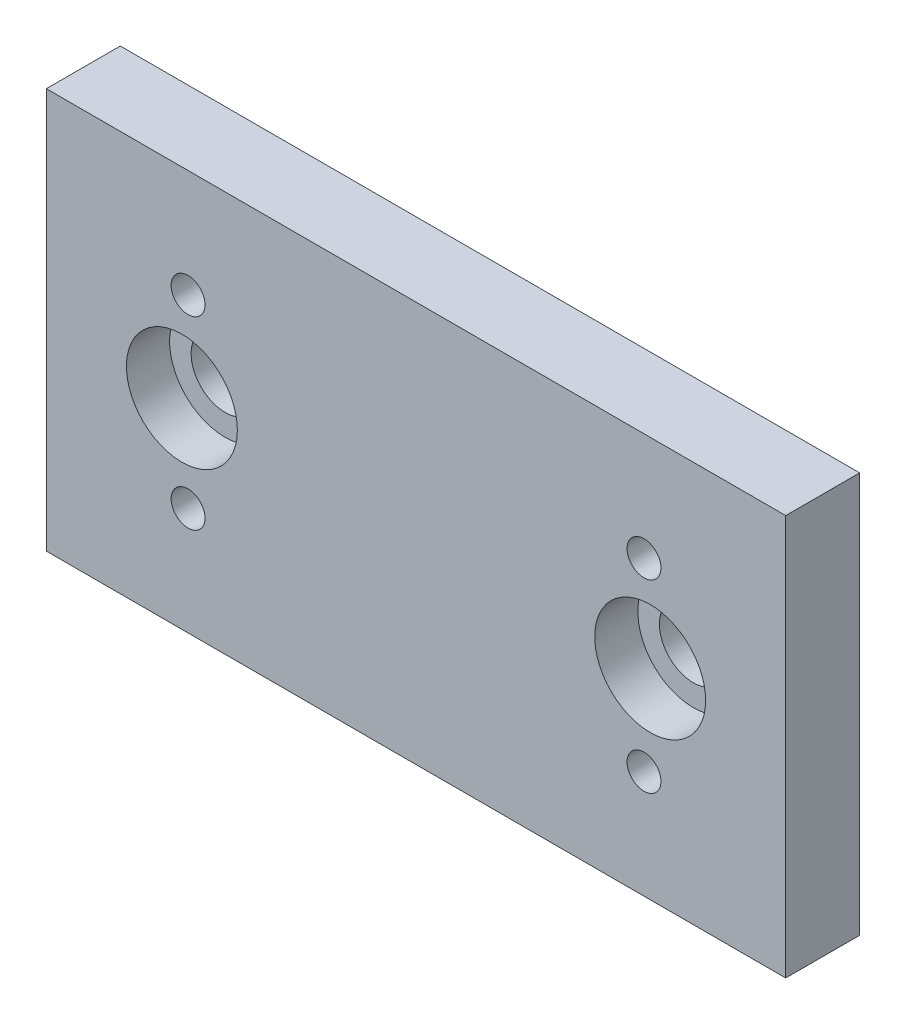
from build123d import *

# Parameters (mm, degrees)
SKETCH1_W                                        = 120
SKETCH1_H                                        = 65
BOSS_EXTRUDE1_DEPTH                              = 12
HOLE_FOR_TORX_SOCKET_CAP_SCREW1_D                = 11
HOLE_FOR_TORX_SOCKET_CAP_SCREW1_CBORE_D          = 18
HOLE_FOR_TORX_SOCKET_CAP_SCREW1_CBORE_DEPTH      = 7
HOLE_FOR_SOCKET_HEAD_CAP_SCREW_TYPE2_D           = 5.5
HOLE_FOR_SOCKET_HEAD_CAP_SCREW_TYPE2_CBORE_D     = 10
HOLE_FOR_SOCKET_HEAD_CAP_SCREW_TYPE2_CBORE_DEPTH = 5.7


with BuildPart() as part:
    # Sketch1 → Boss-Extrude1 (new body)
    with BuildSketch(Plane.XY):
        Rectangle(SKETCH1_W, SKETCH1_H)
    extrude(amount=BOSS_EXTRUDE1_DEPTH)

    # Hole for Torx socket cap screw1 (through all)
    with Locations(Plane.XY.offset(12)):
        with Locations((-38, 0), (38, 0)):
            CounterBoreHole(HOLE_FOR_TORX_SOCKET_CAP_SCREW1_D / 2, HOLE_FOR_TORX_SOCKET_CAP_SCREW1_CBORE_D / 2, HOLE_FOR_TORX_SOCKET_CAP_SCREW1_CBORE_DEPTH)

    # Hole for socket head cap screw, type2 (through all)
    with Locations(Plane(origin=(0, 0, 0), x_dir=(-1, 0, 0), z_dir=(0, 0, -1))):
        with Locations((-37, 15), (-37, -15), (37, -15), (37, 15)):
            CounterBoreHole(HOLE_FOR_SOCKET_HEAD_CAP_SCREW_TYPE2_D / 2, HOLE_FOR_SOCKET_HEAD_CAP_SCREW_TYPE2_CBORE_D / 2, HOLE_FOR_SOCKET_HEAD_CAP_SCREW_TYPE2_CBORE_DEPTH)


solid = part.part
